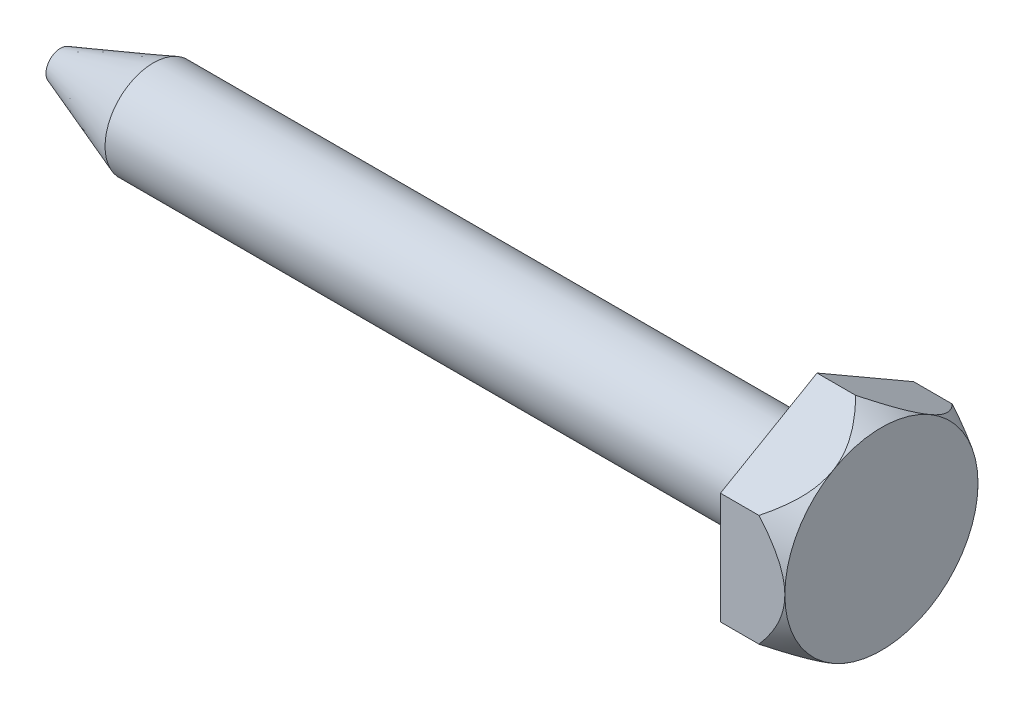
SolidWorks part; units mm, degrees
ref_plane "Front Plane" through (0, 0, 0) normal (0, 0, 1) x (1, 0, 0)
ref_plane "Top Plane" through (0, 0, 0) normal (0, 1, 0) x (1, 0, 0)
ref_plane "Right Plane" through (0, 0, 0) normal (1, 0, 0) x (0, 0, -1)
other "Configuration Table"
sketch "Sketch1" plane through (0, 0, 0) normal (1, 0, 0) x (0, 0, -1)
  line L1 (0, -6.9282) -> (6, -3.4641)
  line L2 (6, -3.4641) -> (6, 3.4641)
  line L3 (6, 3.4641) -> (0, 6.9282)
  line L4 (0, 6.9282) -> (-6, 3.4641)
  line L5 (-6, 3.4641) -> (-6, -3.4641)
  line L6 (-6, -3.4641) -> (0, -6.9282)
  circle A0 centre (0, 0) radius 6 construction
  dimension "D1" = 12
extrude "Boss-Extrude1" add sketch "Sketch1" along normal blind 4
sketch "Sketch2" plane through (4, 0, 0) normal (1, 0, 0) x (0, 0, -1)
  line L0 (0, 6.9282) -> (-6, 3.4641) construction
  circle A0 centre (0, 0) radius 6
extrude "Cut-Extrude1" cut sketch "Sketch2" against normal blind 20 draft 30 flip side to cut
sketch "Sketch3" plane through (0, 0, 0) normal (0, 0, 1) x (1, 0, 0)
  line L0 (-32.1994, 0) -> (13.5275, 0) construction
  line L1 (0, 0) -> (0, 3)
  line L2 (0, 6.9282) -> (0, 3.4641) construction
  line L3 (0, 3) -> (-41.2303, 3)
  line L4 (-41.2303, 3) -> (-47, 0.9)
  line L5 (-47, 0.9) -> (-47, 0)
  line L6 (-47, 0) -> (0, 0)
  dimension "D1" = 47
  dimension "D2" = 6
  dimension "D3" = 1.8
  dimension "D4" = 20
revolve "Revolve1" add sketch "Sketch3" angle 360 about L0
cosmetic thread "Cosmetic Thread1" parameters "D2"=4.917
